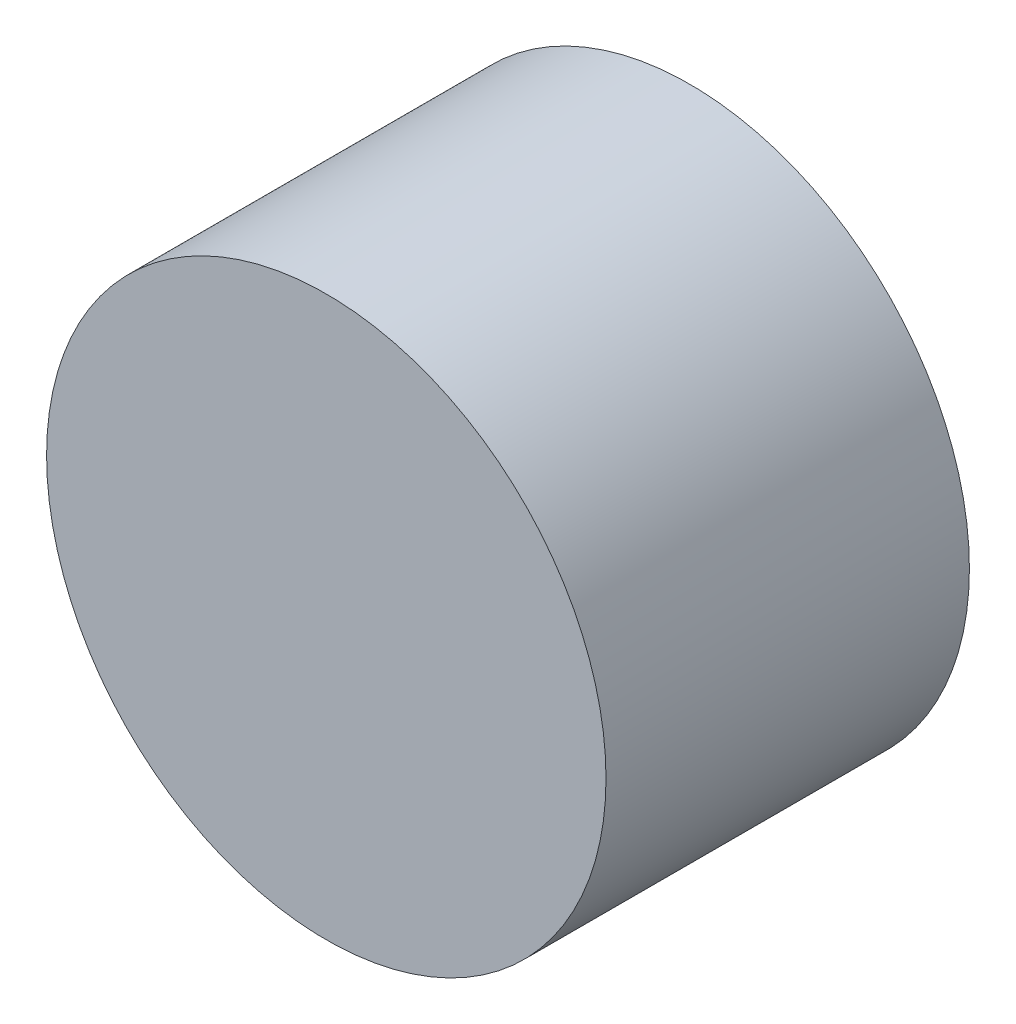
SolidWorks part; units mm, degrees
ref_plane "Front Plane" through (0, 0, 0) normal (0, 0, 1) x (1, 0, 0)
ref_plane "Top Plane" through (0, 0, 0) normal (0, 1, 0) x (1, 0, 0)
ref_plane "Right Plane" through (0, 0, 0) normal (1, 0, 0) x (0, 0, -1)
sketch "Sketch1" plane through (0, 0, 0) normal (0, 0, 1) x (1, 0, 0)
  circle A0 centre (-17.0558, 0) radius 7.6974
extrude "Boss-Extrude1" add sketch "Sketch1" along normal blind 10
